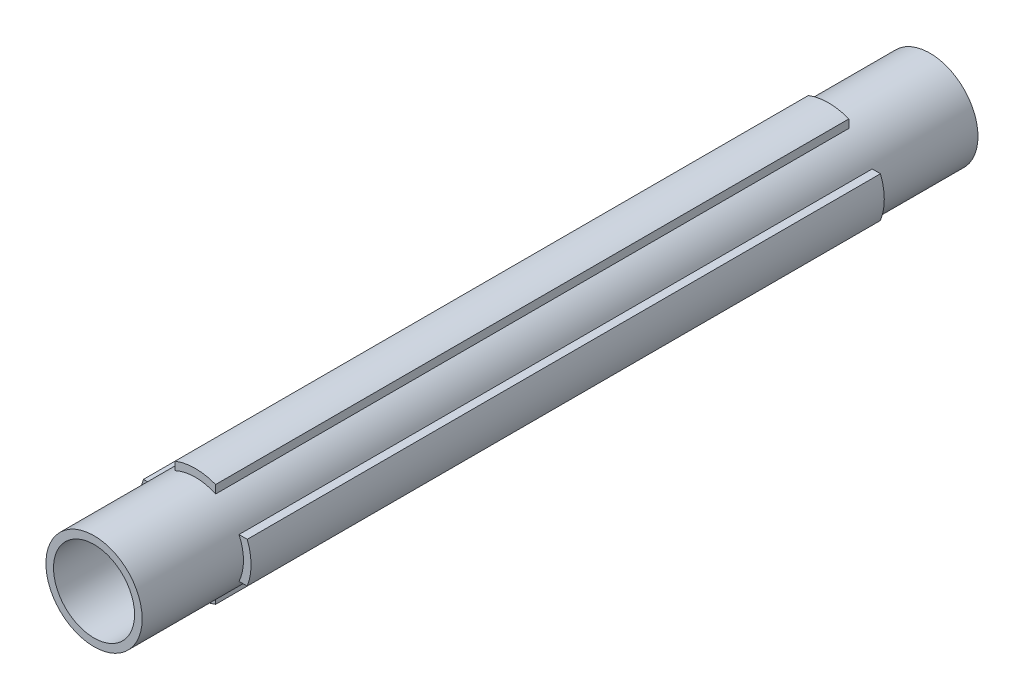
from build123d import *

# Parameters (mm, degrees)
EXTRUDE_1_DEPTH      = 125
EXTRUDE_2_DEPTH      = 20
EXTRUDE_2_DEPTH_BACK = 145
SKETCH_2_R           = 9.5
SKETCH_2_R_2         = 8


with BuildPart() as part:
    # 草图1 → 凸台-拉伸1 (new body)
    with BuildSketch(Plane.XY):
        with BuildLine():
            Line((-4, 10.246950766), (-4, 8.61684397))
            ThreePointArc((-4, 8.61684397), (-6.717514421, 6.717514421), (-8.61684397, 4))
            Line((-8.61684397, 4), (-10.246950766, 4))
            ThreePointArc((-10.246950766, 4), (-11, 0), (-10.246950766, -4))
            Line((-10.246950766, -4), (-8.61684397, -4))
            ThreePointArc((-8.61684397, -4), (-6.717514421, -6.717514421), (-4, -8.61684397))
            Line((-4, -8.61684397), (-4, -10.246950766))
            ThreePointArc((-4, -10.246950766), (0, -11), (4, -10.246950766))
            Line((4, -10.246950766), (4, -8.61684397))
            ThreePointArc((4, -8.61684397), (6.717514421, -6.717514421), (8.61684397, -4))
            Line((8.61684397, -4), (10.246950766, -4))
            ThreePointArc((10.246950766, -4), (11, 0), (10.246950766, 4))
            Line((10.246950766, 4), (8.61684397, 4))
            ThreePointArc((8.61684397, 4), (6.717514421, 6.717514421), (4, 8.61684397))
            Line((4, 8.61684397), (4, 10.246950766))
            ThreePointArc((4, 10.246950766), (0, 11), (-4, 10.246950766))
        make_face()
        with BuildLine():
            Line((-2.5, 9.16515139), (-2.5, 7.599342077))
            ThreePointArc((-2.5, 7.599342077), (-5.656854249, 5.656854249), (-7.599342077, 2.5))
            Line((-7.599342077, 2.5), (-9.16515139, 2.5))
            ThreePointArc((-9.16515139, 2.5), (-9.5, 0), (-9.16515139, -2.5))
            Line((-9.16515139, -2.5), (-7.599342077, -2.5))
            ThreePointArc((-7.599342077, -2.5), (-5.656854249, -5.656854249), (-2.5, -7.599342077))
            Line((-2.5, -7.599342077), (-2.5, -9.16515139))
            ThreePointArc((-2.5, -9.16515139), (0, -9.5), (2.5, -9.16515139))
            Line((2.5, -9.16515139), (2.5, -7.599342077))
            ThreePointArc((2.5, -7.599342077), (5.656854249, -5.656854249), (7.599342077, -2.5))
            Line((7.599342077, -2.5), (9.16515139, -2.5))
            ThreePointArc((9.16515139, -2.5), (9.5, 0), (9.16515139, 2.5))
            Line((9.16515139, 2.5), (7.599342077, 2.5))
            ThreePointArc((7.599342077, 2.5), (5.656854249, 5.656854249), (2.5, 7.599342077))
            Line((2.5, 7.599342077), (2.5, 9.16515139))
            ThreePointArc((2.5, 9.16515139), (0, 9.5), (-2.5, 9.16515139))
        make_face(mode=Mode.SUBTRACT)
    extrude(amount=EXTRUDE_1_DEPTH)

    # 草图2 → 凸台-拉伸2 (add, two sides: drawn at the far end of the back side and taken through both)
    with BuildSketch(Plane.XY.offset(125).offset(-EXTRUDE_2_DEPTH_BACK)):
        Circle(SKETCH_2_R)
        Circle(SKETCH_2_R_2, mode=Mode.SUBTRACT)
    extrude(amount=EXTRUDE_2_DEPTH + EXTRUDE_2_DEPTH_BACK)


solid = part.part
